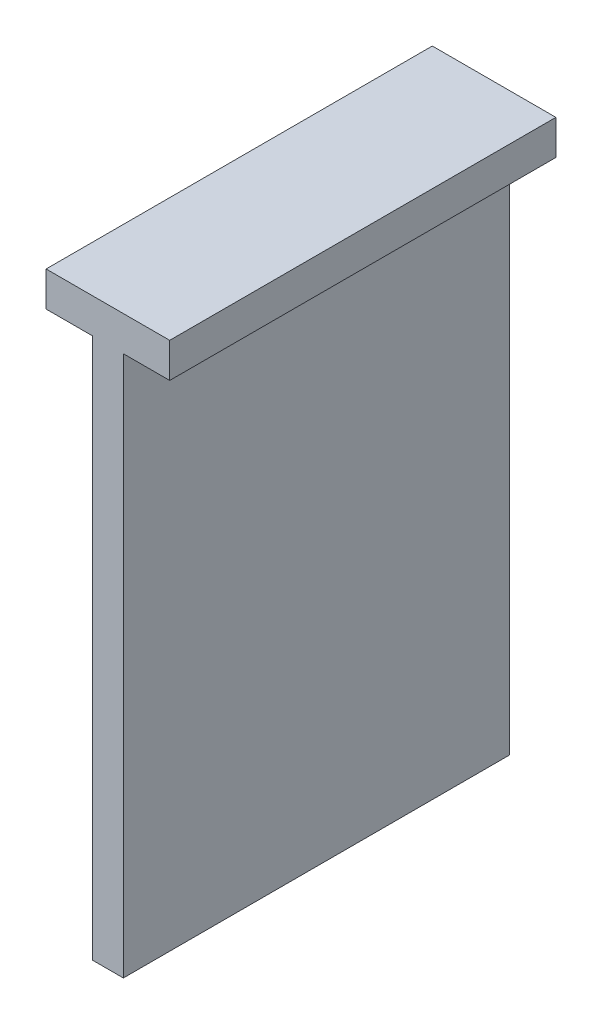
SolidWorks part; units mm, degrees
ref_plane "前视基准面" through (0, 0, 0) normal (0, 0, 1) x (1, 0, 0)
ref_plane "上视基准面" through (0, 0, 0) normal (0, 1, 0) x (1, 0, 0)
ref_plane "右视基准面" through (0, 0, 0) normal (1, 0, 0) x (0, 0, -1)
sketch "草图1" plane through (0, 0, 0) normal (0, 0, 1) x (1, 0, 0)
  line L6 (-32.0398, -6.5119) -> (-32.0398, -120.0953)
  line L8 (-24.0398, -6.5119) -> (-24.0398, -120.0953)
  line L15 (-44.0398, 2.4881) -> (-44.0398, -6.5119)
  line L16 (-44.0398, -6.5119) -> (-32.0398, -6.5119)
  line L18 (-12.0398, 2.4881) -> (-12.0398, -6.5119)
  line L19 (-12.0398, -6.5119) -> (-24.0398, -6.5119)
  line L21 (-44.0398, 2.4881) -> (-12.0398, 2.4881)
  line L22 (-32.0398, -120.0953) -> (-32.0398, -146.5119)
  line L23 (-32.0398, -146.5119) -> (-24.0398, -146.5119)
  line L24 (-24.0398, -120.0953) -> (-24.0398, -146.5119)
  dimension "D1" = 12
  dimension "D2" = 12
  dimension "D3" = 9
  dimension "D4" = 140
  dimension "D5" = 32
extrude "凸台-拉伸1" add sketch "草图1" along normal blind 100
